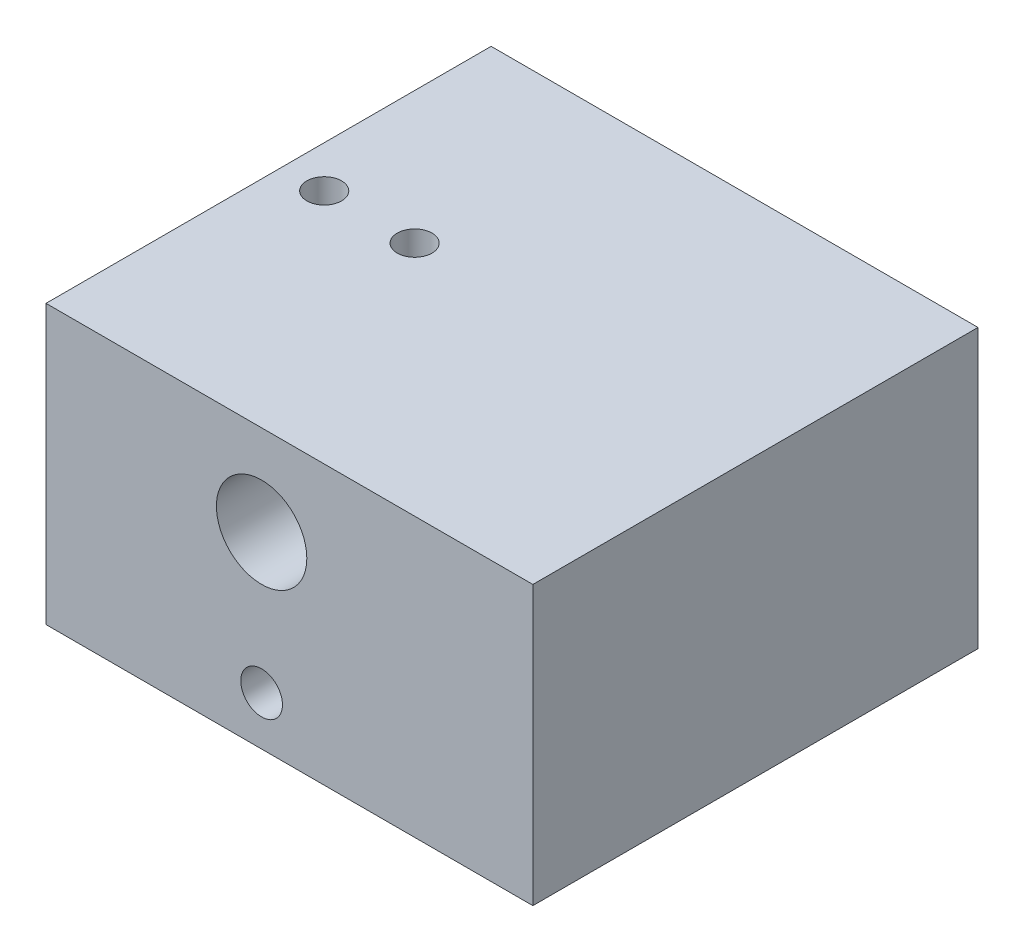
from build123d import *

# Parameters (mm, degrees)
SKETCH1_W             = 35
SKETCH1_H             = 32
BOSS_EXTRUDE1_DEPTH   = 20
CUT_EXTRUDE2_REACH    = 43.596
SKETCH3_R             = 3.25
SKETCH3_R_2           = 1.5
SKETCH4_R             = 1
CUT_EXTRUDE3_DEPTH    = 2
M3_TAPPED_HOLE1_D     = 2.5
M3_TAPPED_HOLE1_DEPTH = 7.5
M3_TAPPED_HOLE1_TIP   = 0.751075774


with BuildPart() as part:
    # Sketch1 → Boss-Extrude1 (new body)
    with BuildSketch(Plane(origin=(0, 0, 0), x_dir=(1, 0, 0), z_dir=(0, 1, 0))):
        Rectangle(SKETCH1_W, SKETCH1_H)
    extrude(amount=BOSS_EXTRUDE1_DEPTH)

    # Sketch3 → Cut-Extrude2 (cut, up to next)
    with BuildSketch(Plane.XY.offset(16), mode=Mode.PRIVATE) as cut_extrude2_sk1:
        with Locations((-2, 13.5)):
            Circle(SKETCH3_R)
    cut_extrude2_tool1 = extrude(cut_extrude2_sk1.sketch, amount=-CUT_EXTRUDE2_REACH, mode=Mode.PRIVATE) & part.part
    # Sketch3 → Cut-Extrude2 (cut, up to next)
    with BuildSketch(Plane.XY.offset(16), mode=Mode.PRIVATE) as cut_extrude2_sk2:
        with Locations((-2, 3.5)):
            Circle(SKETCH3_R_2)
    cut_extrude2_tool2 = extrude(cut_extrude2_sk2.sketch, amount=-CUT_EXTRUDE2_REACH, mode=Mode.PRIVATE) & part.part
    add(cut_extrude2_tool1.solids().sort_by_distance((-2, 13.5, 16))[0], mode=Mode.SUBTRACT)
    add(cut_extrude2_tool2.solids().sort_by_distance((-2, 3.5, 16))[0], mode=Mode.SUBTRACT)

    # Sketch4 → Cut-Extrude3 (cut)
    with BuildSketch(Plane(origin=(0, 20, 0), x_dir=(1, 0, 0), z_dir=(0, 1, 0))):
        with Locations(Location((-8, 1, 0), (0, 0, 270))):
            Circle(SKETCH4_R)
        with Locations(Location((-14.5, 1, 0), (0, 0, 270))):
            Circle(SKETCH4_R)
    extrude(amount=-CUT_EXTRUDE3_DEPTH, mode=Mode.SUBTRACT)

    # M3 Tapped Hole1
    with Locations(Plane(origin=(0, 20, 0), x_dir=(1, 0, 0), z_dir=(0, 1, 0))):
        with Locations((-8, 1), (-14.5, 1)):
            Hole(M3_TAPPED_HOLE1_D / 2, depth=M3_TAPPED_HOLE1_DEPTH)
            with Locations((0, 0, -(M3_TAPPED_HOLE1_DEPTH + M3_TAPPED_HOLE1_TIP / 2))):  # 118° drill point
                Cone(0, M3_TAPPED_HOLE1_D / 2, M3_TAPPED_HOLE1_TIP, mode=Mode.SUBTRACT)


solid = part.part
